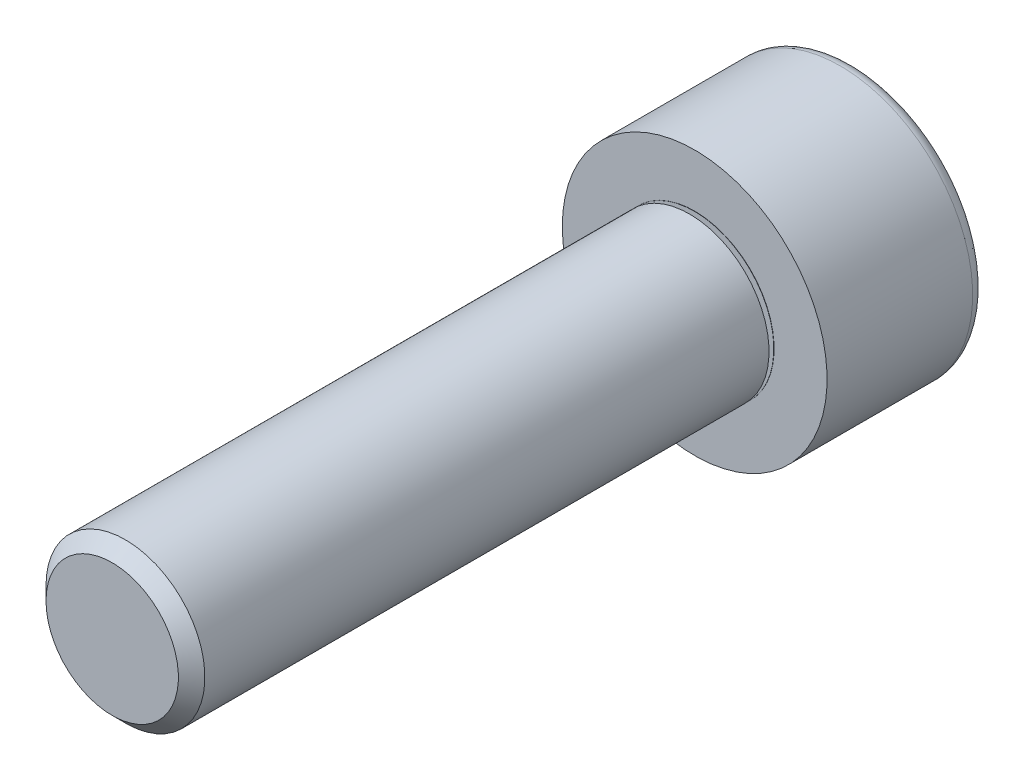
SolidWorks part; units mm, degrees
ref_plane "Front" through (0, 0, 0) normal (0, 0, 1) x (1, 0, 0)
ref_plane "Top" through (0, 0, 0) normal (0, 1, 0) x (1, 0, 0)
ref_plane "Right" through (0, 0, 0) normal (1, 0, 0) x (0, 0, -1)
sketch "Logo3_Revol_Axis" plane through (0, 0, 0) normal (0, 1, 0) x (1, 0, 0)
  line L0 (0, -43.5172) -> (0, 43.5172) construction
sketch "Logo3_bib1" plane through (0, 0, 0) normal (0, -1, 0) x (-1, 0, 0)
  line L0 (0, -22) -> (0, 6)
  line L1 (0, 6) -> (4.5, 6)
  line L2 (5, 5.5) -> (5, 0)
  line L3 (5, 0) -> (3, 0)
  line L4 (3, 0) -> (3, -0.01)
  line L5 (3, -21.5) -> (2.5, -22)
  line L6 (2.5, -22) -> (0, -22)
  line L7 (3, -0.01) -> (2.6134, -0.01)
  line L8 (2.6066, -0.0488) -> (3, -0.192)
  line L9 (3, -0.192) -> (3, -21.5)
  line L10 (0, 10.5852) -> (0, -63.2873) construction
  arc A0 (4.5, 6) -> (5, 5.5) centre (4.5, 5.5) cw
  arc A1 (2.6134, -0.01) -> (2.6066, -0.0488) centre (2.6134, -0.03) ccw
  point P17 (2.5, -0.01)
revolve "Revolve1" add sketch "Logo3_bib1" angle 360 about L10
cosmetic thread "Cosmetic Thread1" parameters "D2"=5
sketch "Logo3_bib2" plane through (0, 0, -6) normal (0, 0, -1) x (1, 0, 0)
  line L1 (2.8868, 0) -> (1.4434, 2.5)
  line L2 (1.4434, 2.5) -> (-1.4434, 2.5)
  line L3 (-1.4434, 2.5) -> (-2.8868, 0)
  line L4 (-2.8868, 0) -> (-1.4434, -2.5)
  line L5 (-1.4434, -2.5) -> (1.4434, -2.5)
  line L6 (1.4434, -2.5) -> (2.8868, 0)
  circle A0 centre (0, 0) radius 2.5 construction
extrude "Cut-Extrude1" cut sketch "Logo3_bib2" against normal blind 2.5
equation "\"DIA2@XZQB7_bib1\" = \"XZQB7_d1-pas@XZQB7_bib1\""
equation "\"LGT1@XZQB7_bib1\" = \"XZQB7_d1@XZQB7_bib1\""
equation "\"D1@Cut-Extrude1\" = \"XZQB7_c1@XZQB7_bib2\"/2."
equation "\"D2@Cosmetic Thread1\" = \"XZQB7_d1-pas@XZQB7_bib1\""
